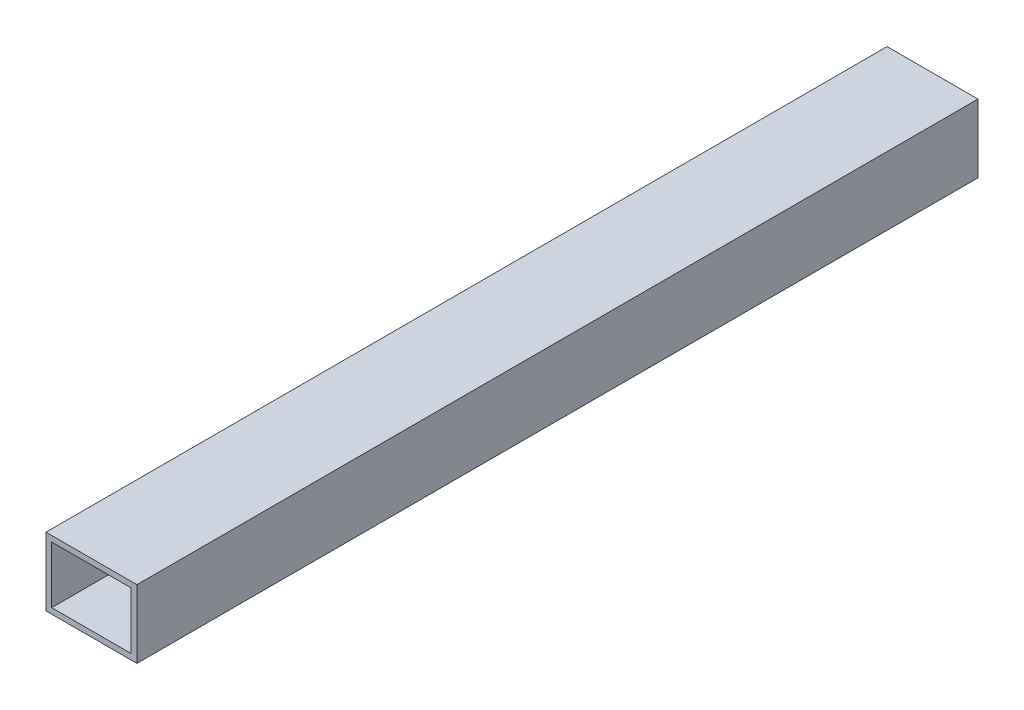
from build123d import *

# Parameters (mm, degrees)
SKETCH_1_W          = 80
SKETCH_1_H          = 60
SKETCH_1_W_2        = 74
SKETCH_1_H_2        = 54
EXTRUDE_1_DEPTH     = 740
SKETCH_3_W          = 80
SKETCH_3_H          = 60
CUT_EXTRUDE_1_DEPTH = 25
SKETCH_4_W          = 80
SKETCH_4_H          = 60
CUT_EXTRUDE_2_DEPTH = 25
SKETCH_5_W          = 80
SKETCH_5_H          = 60
SKETCH_5_W_2        = 74
SKETCH_5_H_2        = 54
EXTRUDE_2_DEPTH     = 25
SKETCH_6_W          = 80
SKETCH_6_H          = 60
SKETCH_6_W_2        = 74
SKETCH_6_H_2        = 54
EXTRUDE_3_DEPTH     = 25
SKETCH_7_W          = 45
SKETCH_7_H          = 5
CUT_EXTRUDE_3_DEPTH = 80
EXTRUDE_4_DEPTH     = 45
EXTRUDE_5_DEPTH     = 45
SKETCH_10_W         = 74
SKETCH_10_H         = 54
SKETCH_10_W_2       = 70
SKETCH_10_H_2       = 50
EXTRUDE_6_DEPTH     = 740


with BuildPart() as part:
    # 草图1 → 凸台-拉伸1 (new body)
    with BuildSketch(Plane.XY):
        with Locations((40, -30)):
            Rectangle(SKETCH_1_W, SKETCH_1_H)
        with Locations((40, -30)):
            Rectangle(SKETCH_1_W_2, SKETCH_1_H_2, mode=Mode.SUBTRACT)
    extrude(amount=EXTRUDE_1_DEPTH)

    # 草图3 → 切除-拉伸1 (cut)
    with BuildSketch(Plane.XY.offset(740)):
        with Locations((40, -30)):
            Rectangle(SKETCH_3_W, SKETCH_3_H)
    extrude(amount=-CUT_EXTRUDE_1_DEPTH, mode=Mode.SUBTRACT)

    # 草图4 → 切除-拉伸2 (cut)
    with BuildSketch(Plane(origin=(0, 0, 0), x_dir=(-1, 0, 0), z_dir=(0, 0, -1))):
        with Locations((-40, -30)):
            Rectangle(SKETCH_4_W, SKETCH_4_H)
    extrude(amount=-CUT_EXTRUDE_2_DEPTH, mode=Mode.SUBTRACT)

    # 草图5 → 凸台-拉伸2 (add)
    with BuildSketch(Plane.XY.offset(715)):
        with Locations((40, -30)):
            Rectangle(SKETCH_5_W, SKETCH_5_H)
        with Locations((40, -30)):
            Rectangle(SKETCH_5_W_2, SKETCH_5_H_2, mode=Mode.SUBTRACT)
    extrude(amount=EXTRUDE_2_DEPTH)

    # 草图6 → 凸台-拉伸3 (add)
    with BuildSketch(Plane(origin=(0, 0, 25), x_dir=(-1, 0, 0), z_dir=(0, 0, -1))):
        with Locations((-40, -30)):
            Rectangle(SKETCH_6_W, SKETCH_6_H)
        with Locations((-40, -30)):
            Rectangle(SKETCH_6_W_2, SKETCH_6_H_2, mode=Mode.SUBTRACT)
    extrude(amount=EXTRUDE_3_DEPTH)

    # 草图7 → 切除-拉伸3 (cut)
    with BuildSketch(Plane(origin=(80, 0, 0), x_dir=(0, 0, -1), z_dir=(1, 0, 0))):
        with Locations((-717.5, -57.5)):
            Rectangle(SKETCH_7_W, SKETCH_7_H)
        with Locations((-22.5, -57.5)):
            Rectangle(SKETCH_7_W, SKETCH_7_H)
    extrude(amount=-CUT_EXTRUDE_3_DEPTH, mode=Mode.SUBTRACT)

    # 草图8 → 凸台-拉伸4 (add)
    with BuildSketch(Plane(origin=(0, 0, 45), x_dir=(-1, 0, 0), z_dir=(0, 0, -1))):
        Polygon((-3, -55), (-3, -57), (-77, -57), (-77, -55), (-80, -55), (-80, -60), (0, -60), (0, -55), align=None)
    extrude(amount=EXTRUDE_4_DEPTH)

    # 草图9 → 凸台-拉伸5 (add)
    with BuildSketch(Plane.XY.offset(695)):
        Polygon((3, -57), (3, -55), (0, -55), (0, -60), (80, -60), (80, -55), (77, -55), (77, -57), align=None)
    extrude(amount=EXTRUDE_5_DEPTH)

    # 草图10 → 凸台-拉伸6 (add)
    with BuildSketch(Plane(origin=(0, 0, 0), x_dir=(-1, 0, 0), z_dir=(0, 0, -1))):
        with Locations((-40, -30)):
            Rectangle(SKETCH_10_W, SKETCH_10_H)
        with Locations((-40, -30)):
            Rectangle(SKETCH_10_W_2, SKETCH_10_H_2, mode=Mode.SUBTRACT)
    extrude(amount=-EXTRUDE_6_DEPTH)


solid = part.part
